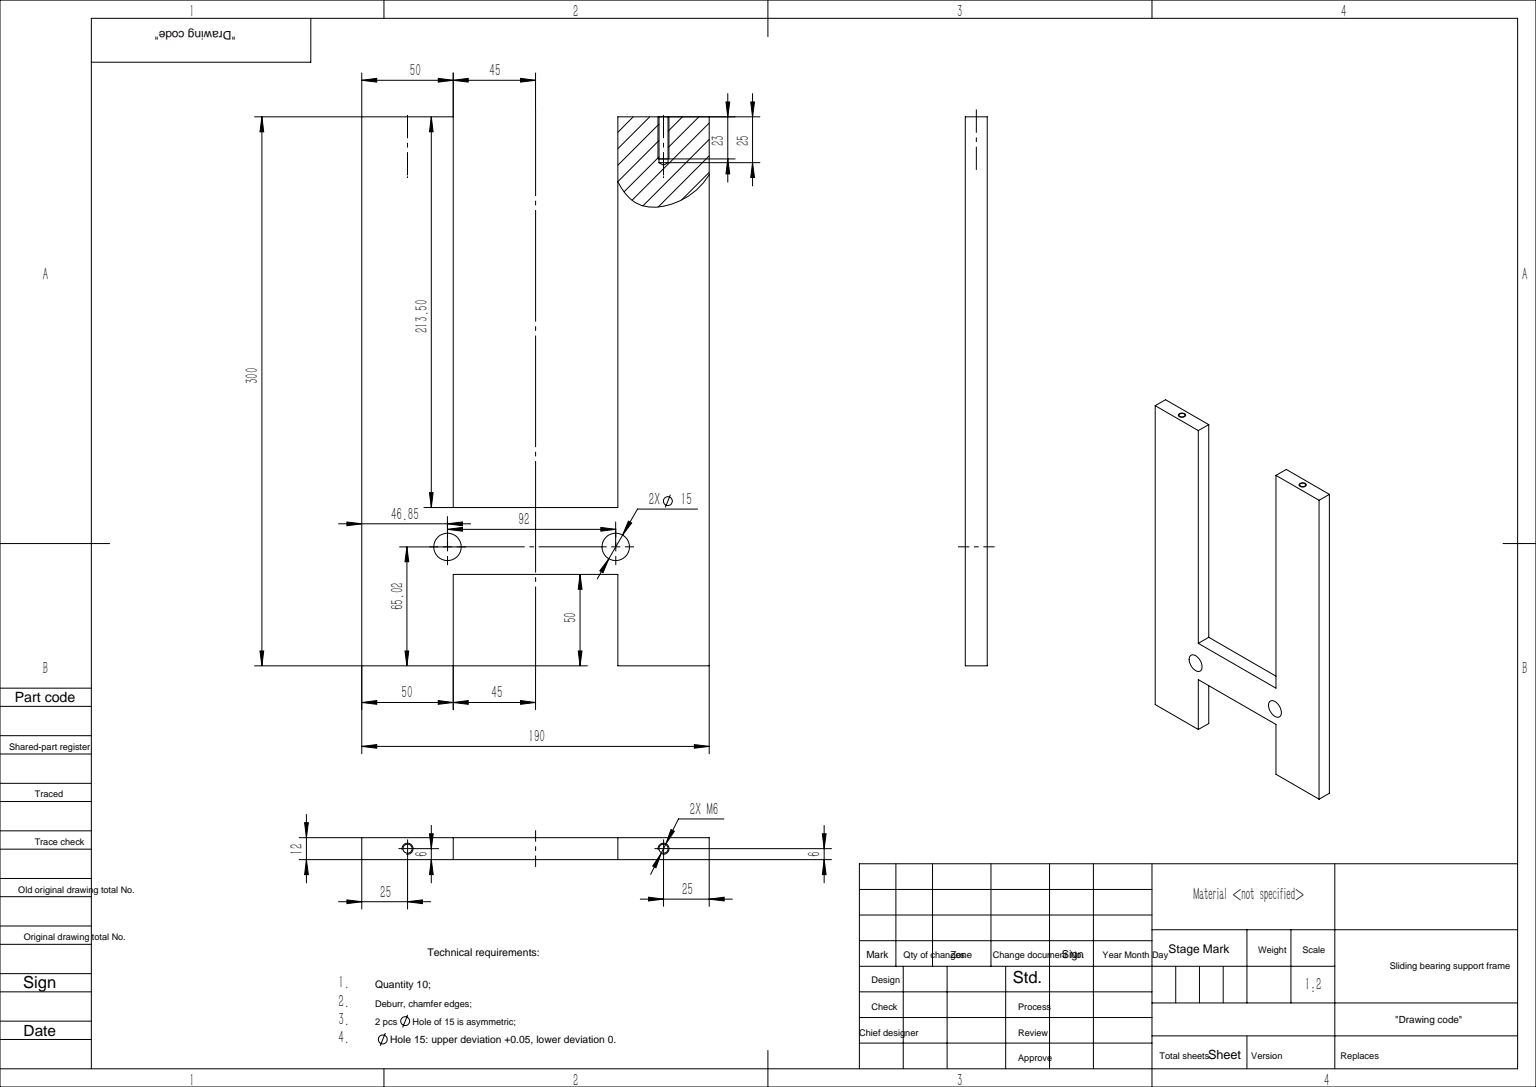
from build123d import *

# Parameters (mm, degrees)
SKETCH_1_R             = 7.5
EXTRUDE_1_DEPTH        = 6
HOLE_WIZARD_M6_1_D     = 5
HOLE_WIZARD_M6_1_DEPTH = 25
HOLE_WIZARD_M6_1_TIP   = 1.443375673


with BuildPart() as part:
    # 草图1 → 凸台-拉伸1 (new, symmetric)
    with BuildSketch(Plane(origin=(0, 0, -465), x_dir=(-1, 0, 0), z_dir=(0, 0, -1))):
        Polygon((-557.085724054, 1805.000303929), (-557.085724054, 1591.500303929), (-647.085724054, 1591.500303929), (-647.085724054, 1805.000303929), (-697.085724054, 1805.000303929), (-697.085724054, 1505.000303929), (-647.085724054, 1505.000303929), (-647.085724054, 1555.000303929), (-557.085724054, 1555.000303929), (-557.085724054, 1505.000303929), (-507.085724054, 1505.000303929), (-507.085724054, 1805.000303929), align=None)
        with Locations((-553.939078063, 1570.019037425)):
            Circle(SKETCH_1_R, mode=Mode.SUBTRACT)
        with Locations((-645.939078063, 1570.019037425)):
            Circle(SKETCH_1_R, mode=Mode.SUBTRACT)
    extrude(amount=EXTRUDE_1_DEPTH, both=True)

    # M6 螺纹孔1
    with Locations(Plane(origin=(0, 1805.000303929, 0), x_dir=(1, 0, 0), z_dir=(0, 1, 0))):
        with Locations((672.085724054, 465), (532.085724054, 465)):
            Hole(HOLE_WIZARD_M6_1_D / 2, depth=HOLE_WIZARD_M6_1_DEPTH)
            with Locations((0, 0, -(HOLE_WIZARD_M6_1_DEPTH + HOLE_WIZARD_M6_1_TIP / 2))):  # 120° drill point
                Cone(0, HOLE_WIZARD_M6_1_D / 2, HOLE_WIZARD_M6_1_TIP, mode=Mode.SUBTRACT)


solid = part.part
